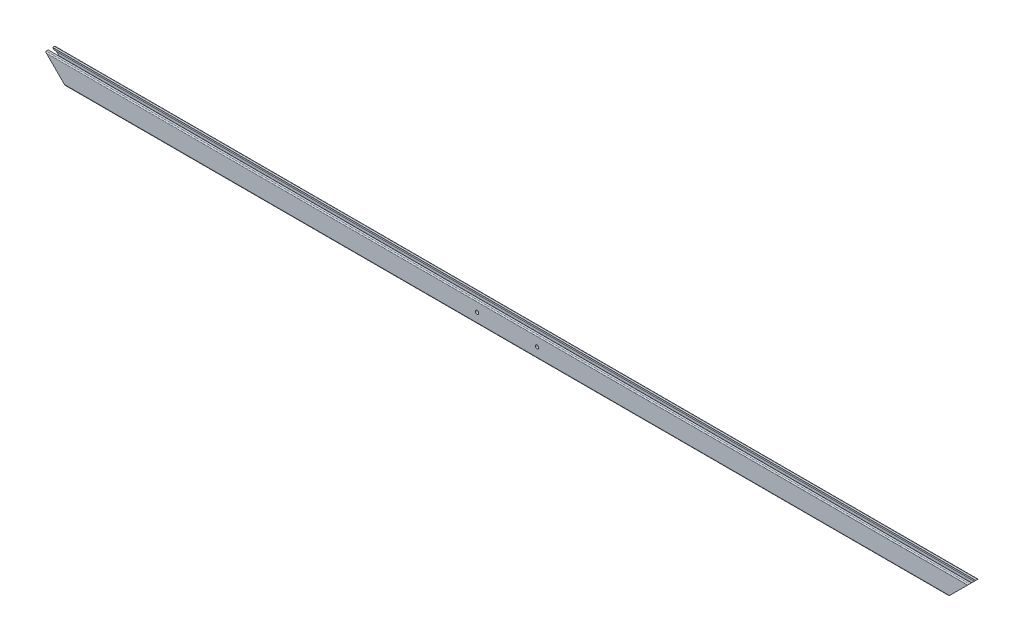
from build123d import *

# Parameters (mm, degrees)
SKETCH11_R          = 2.5
MEMBER_1_DEPTH      = 1386
CUT_EXTRUDE_1_DEPTH = 694.324599304
HOLE_WIZARD_M6_1_D  = 5


with BuildPart() as part:
    # Sketch11 → Member 1 (new body)
    with BuildSketch(Plane(origin=(-693, 0, 0), x_dir=(0, 0, -1), z_dir=(1, 0, 0))):
        with BuildLine():
            Line((-6, -15), (-3.25, -15))
            Line((-3.25, -15), (-3.25, -12.7))
            Line((-3.25, -12.7), (-5, -12.7))
            Line((-5, -12.7), (-5, -7))
            ThreePointArc((-5, -7), (0, -4.31662479), (5, -7))
            Line((5, -7), (5, -12.7))
            Line((5, -12.7), (3.25, -12.7))
            Line((3.25, -12.7), (3.25, -15))
            Line((3.25, -15), (6, -15))
            ThreePointArc((6, -15), (7.060660172, -14.560660172), (7.5, -13.5))
            Line((7.5, -13.5), (7.5, 13.5))
            ThreePointArc((7.5, 13.5), (7.060660172, 14.560660172), (6, 15))
            Line((6, 15), (3.25, 15))
            Line((3.25, 15), (3.25, 12.7))
            Line((3.25, 12.7), (5, 12.7))
            Line((5, 12.7), (5, 7))
            ThreePointArc((5, 7), (0, 4.31662479), (-5, 7))
            Line((-5, 7), (-5, 12.7))
            Line((-5, 12.7), (-3.25, 12.7))
            Line((-3.25, 12.7), (-3.25, 15))
            Line((-3.25, 15), (-6, 15))
            ThreePointArc((-6, 15), (-7.060660172, 14.560660172), (-7.5, 13.5))
            Line((-7.5, 13.5), (-7.5, -13.5))
            ThreePointArc((-7.5, -13.5), (-7.060660172, -14.560660172), (-6, -15))
        make_face()
        Circle(SKETCH11_R, mode=Mode.SUBTRACT)
    extrude(amount=MEMBER_1_DEPTH)

    # 草图4 → 切除-拉伸1 (cut, through all)
    with BuildSketch(Plane.XY.offset(7.5)):
        Polygon((-693, 15), (-663, -15), (-693, -15), align=None)
        Polygon((693, -15), (693, 15), (663, -15), align=None)
    extrude(amount=-CUT_EXTRUDE_1_DEPTH, mode=Mode.SUBTRACT)

    # M6 螺纹孔1 (through all)
    with Locations(Plane.XY.offset(7.5)):
        with Locations((-45, 0), (45, 0)):
            Hole(HOLE_WIZARD_M6_1_D / 2)


solid = part.part
